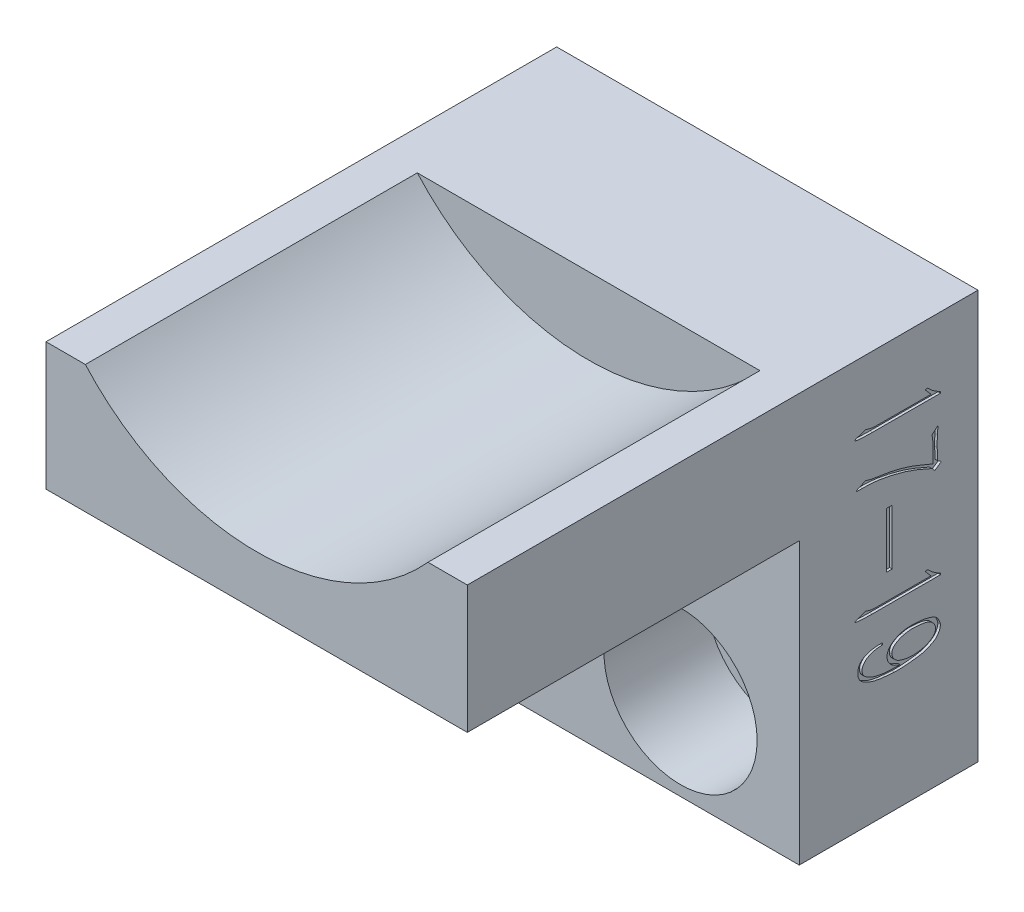
SolidWorks part; units mm, degrees
material "PEEK"
ref_plane "Front Plane" through (0, 0, 0) normal (0, 0, 1) x (1, 0, 0)
ref_plane "Top Plane" through (0, 0, 0) normal (0, 1, 0) x (1, 0, 0)
ref_plane "Right Plane" through (0, 0, 0) normal (1, 0, 0) x (0, 0, -1)
sketch "Sketch1" plane through (0, 0, 0) normal (0, 0, 1) x (1, 0, 0)
  line L1 (-8.25, 8) -> (8.25, 8)
  line L2 (-8.25, 8) -> (-8.25, -8)
  line L3 (-8.25, -8) -> (8.25, -8)
  line L4 (8.25, 8) -> (8.25, -8)
  line L5 (-8.25, 8) -> (8.25, -8) construction
  line L6 (-8.25, -8) -> (8.25, 8) construction
  point P0 (0, 0)
  dimension "D1" = 16.5
  dimension "D2" = 16
extrude "Boss-Extrude1" add sketch "Sketch1" along normal blind 20
sketch "Sketch2" plane through (0, 0, 20) normal (0, 0, 1) x (1, 0, 0)
  line L0 (-8.25, 8) -> (-8.25, -8) construction
  line L1 (-8.25, -8) -> (8.25, -8)
  line L2 (-8.25, -8) -> (-8.25, 3)
  line L3 (-8.25, 3) -> (8.25, 3)
  line L4 (8.25, -8) -> (8.25, 3)
  line L5 (-8.25, -8) -> (8.25, -8) construction
  line L6 (8.25, -8) -> (8.25, 8) construction
  line L7 (8.25, 8) -> (-8.25, 8) construction
  dimension "D1" = 5
extrude "Cut-Extrude1" cut sketch "Sketch2" against normal blind 13
hole_wizard "CBORE for M3 Hex Head Bolt1" positions "Sketch3" profile "Sketch4" counterbore size "M3" standard "GB"
sketch "Sketch3" plane through (0, 0, 7) normal (0, 0, 1) x (1, 0, 0)
  line L0 (-8.25, -8) -> (8.25, -8) construction
  line L1 (-8.25, 3) -> (-8.25, -8) construction
  point P0 (-3.6, -1.4)
  point P2 (3.6, -4.6)
  dimension "D1" = 6.6
  dimension "D2" = 3.4
  dimension "D3" = 4.65
  dimension "D4" = 11.85
sketch "Sketch4" plane through (-3.6, -1.4, 7) normal (1, 0, 0) x (0, -1, 0)
  line L0 (0, 0) -> (0, 8.5515)
  line L1 (0, 8.5515) -> (1.75, 7.5)
  line L2 (1.75, 7.5) -> (1.75, 4)
  line L3 (1.75, 4) -> (3, 4)
  line L4 (3, 4) -> (3, 0)
  line L5 (3, 0) -> (0, 0)
  line L10 (0, 8.5515) -> (-1.75, 7.5) construction
  line L11 (0, -6.35) -> (0, 107.95) construction
  dimension "孔直径" = 3.5
  dimension "孔深度" = 7.5
  dimension "柱形沉头孔直径" = 6
  dimension "柱形沉头孔深度" = 4
  dimension "导头角度" = 118
sketch "Sketch5" plane through (0, 0, 20) normal (0, 0, 1) x (1, 0, 0)
  line L0 (8.25, 8) -> (-8.25, 8) construction
  line L1 (-8.25, -8) -> (8.25, -8) construction
  circle A0 centre (0, 14) radius 9
  point P5 (0, 8)
  dimension "D1" = 18
  dimension "22" = 22
extrude "Cut-Extrude2" cut sketch "Sketch5" against normal blind 13
sketch "Sketch7" plane through (8.25, 0, 0) normal (1, 0, 0) x (0, 0, -1)
  line L0 (-5, 8) -> (-5, -8.7373) construction
  line L1 (-20, 8) -> (0, 8) construction
  line L2 (0, -8) -> (0, 8) construction
  text T0 " 17-19"
  dimension "D1" = 5
extrude "Cut-Extrude4" cut sketch "Sketch7" against normal blind 0.1
equation "\"a\"= \"名称代码\""
equation "\"b\"= \"图号代码\""
